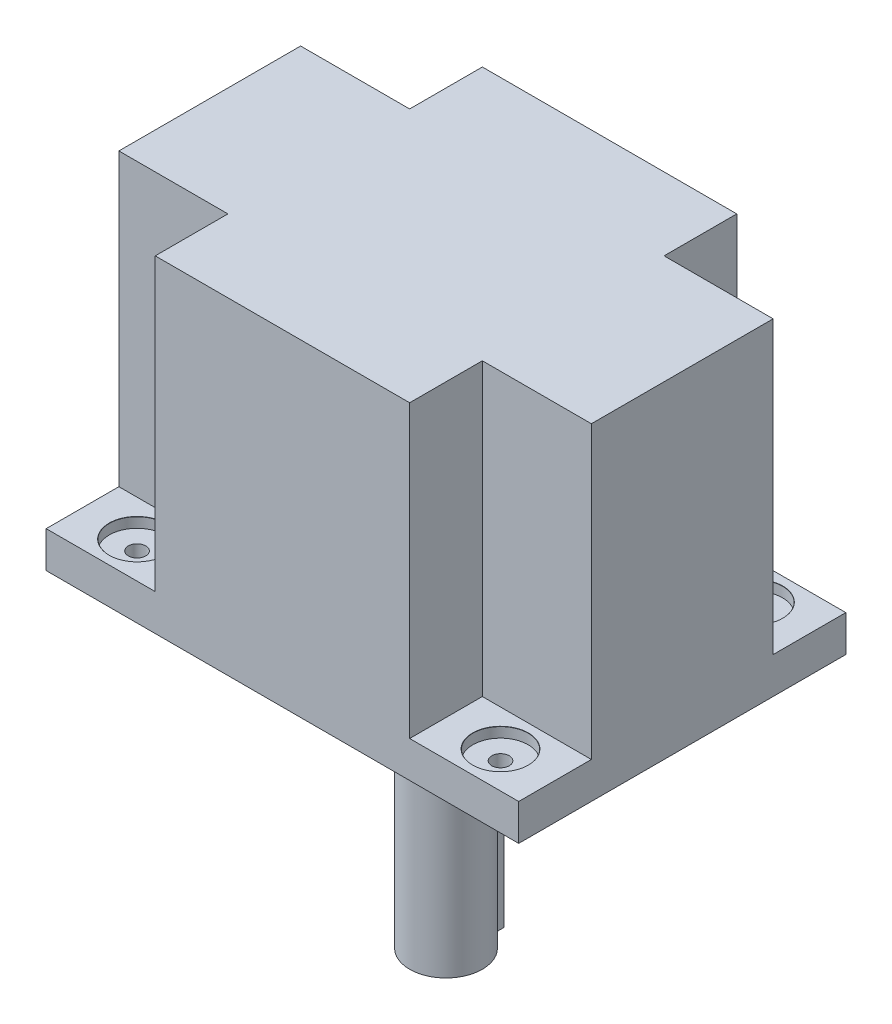
SolidWorks part; units mm, degrees
ref_plane "Front Plane" through (0, 0, 0) normal (0, 0, 1) x (1, 0, 0)
ref_plane "Top Plane" through (0, 0, 0) normal (0, 1, 0) x (1, 0, 0)
ref_plane "Right Plane" through (0, 0, 0) normal (1, 0, 0) x (0, 0, -1)
sketch "Sketch1" plane through (0, 0, 0) normal (0, 1, 0) x (1, 0, 0)
  line L1 (-32.5, -22.5) -> (32.5, -22.5)
  line L2 (-32.5, -22.5) -> (-32.5, 22.5)
  line L3 (-32.5, 22.5) -> (32.5, 22.5)
  line L4 (32.5, -22.5) -> (32.5, 22.5)
  line L5 (-32.5, -22.5) -> (32.5, 22.5) construction
  line L6 (-32.5, 22.5) -> (32.5, -22.5) construction
  point P0 (0, 0)
  dimension "D1" = 65
  dimension "D2" = 45
extrude "Boss-Extrude1" add sketch "Sketch1" along normal blind 45
sketch "Sketch2" plane through (0, 45, 0) normal (0, 1, 0) x (1, 0, 0)
  line L1 (-32.5, 22.5) -> (-17.5, 22.5)
  line L2 (-32.5, 22.5) -> (-32.5, 12.5)
  line L3 (-32.5, 12.5) -> (-17.5, 12.5)
  line L4 (-17.5, 22.5) -> (-17.5, 12.5)
  line L5 (-32.5, -22.5) -> (-17.5, -22.5)
  line L6 (-32.5, -22.5) -> (-32.5, -12.5)
  line L7 (-32.5, -12.5) -> (-17.5, -12.5)
  line L8 (-17.5, -22.5) -> (-17.5, -12.5)
  line L9 (32.5, -22.5) -> (17.5, -22.5)
  line L10 (32.5, -22.5) -> (32.5, -12.5)
  line L11 (32.5, -12.5) -> (17.5, -12.5)
  line L12 (17.5, -22.5) -> (17.5, -12.5)
  line L13 (32.5, 22.5) -> (17.5, 22.5)
  line L14 (32.5, 22.5) -> (32.5, 12.5)
  line L15 (32.5, 12.5) -> (17.5, 12.5)
  line L16 (17.5, 22.5) -> (17.5, 12.5)
  dimension "D1" = 15
  dimension "D2" = 15
  dimension "D3" = 15
  dimension "D4" = 15
  dimension "D5" = 10
  dimension "D6" = 10
  dimension "D7" = 10
  dimension "D8" = 10
extrude "Cut-Extrude1" cut sketch "Sketch2" against normal blind 40
sketch "Sketch3" plane through (0, 0, 0) normal (0, -1, 0) x (1, 0, 0)
  circle A0 centre (0, 0) radius 5
extrude "Boss-Extrude2" add sketch "Sketch3" along normal blind 40
sketch "Sketch4" plane through (0, -40, 0) normal (0, -1, 0) x (1, 0, 0)
  line L0 (0, 0) -> (0, -5)
  line L2 (-1.5, -6.5) -> (1.5, -6.5)
  line L3 (-1.5, -6.5) -> (-1.5, -3.5)
  line L4 (-1.5, -3.5) -> (1.5, -3.5)
  line L5 (1.5, -6.5) -> (1.5, -3.5)
  line L6 (-1.5, -6.5) -> (1.5, -3.5) construction
  line L7 (-1.5, -3.5) -> (1.5, -6.5) construction
  circle A0 centre (0, 0) radius 5 construction
  circle M3 centre (0, 0) radius 5
  dimension "D1" = 3
  dimension "D2" = 3
extrude "Boss-Extrude3" add sketch "Sketch4" against normal up to surface (40 mm away) contours L2 L5 L3 M3 up to face at (0, 0, -5)
sketch "Sketch5" plane through (0, 0, 0) normal (0, -1, 0) x (1, 0, 0)
  circle A0 centre (0, 0) radius 15
extrude "Boss-Extrude4" add sketch "Sketch5" along normal blind 2
hole_wizard "CBORE for M2 Hex Cap Screw1" positions "Sketch6" profile "Sketch8" counterbore size "M2" standard "ISO"
sketch "Sketch6" plane through (0, -40, 0) normal (0, -1, 0) x (-1, 0, 0)
  point P0 (0, 0)
sketch "Sketch8" plane through (0, -40, 0) normal (1, 0, 0) x (0, 0, -1)
  line L0 (0, 0) -> (0, 5.721)
  line L1 (0, 5.721) -> (1.2, 5)
  line L2 (1.2, 5) -> (1.2, 1.4)
  line L3 (1.2, 1.4) -> (3.8095, 1.4)
  line L5 (3.8095, 1.4) -> (3.8095, 0.025)
  line L6 (3.8095, 0.025) -> (3.8345, 0)
  line L7 (3.8345, 0) -> (0, 0)
  line L8 (-3.8095, 0.025) -> (-3.8345, 0) construction
  line L10 (0, 5.721) -> (-1.2, 5) construction
  line L11 (0, -6.35) -> (0, 107.95) construction
  dimension "孔直径" = 2.4
  dimension "孔深度" = 5
  dimension "锥形沉头孔直径" = 7.619
  dimension "锥形沉头孔深度" = 1.4
  dimension "近端锥形沉头孔直径" = 7.669
  dimension "近端锥形沉头孔角度" = 90
  dimension "导头角度" = 118
sketch "Sketch9" plane through (0, -38.6, 0) normal (0, -1, 0) x (1, 0, 0)
  circle A0 centre (0, 0) radius 1.2
sketch "Sketch10" plane through (0, 5, 0) normal (0, 1, 0) x (1, 0, 0)
  line L1 (-25, -17.5) -> (25, -17.5)
  line L2 (-25, -17.5) -> (-25, 17.5)
  line L3 (-25, 17.5) -> (25, 17.5)
  line L4 (25, -17.5) -> (25, 17.5)
  line L5 (-25, -17.5) -> (25, 17.5) construction
  line L6 (-25, 17.5) -> (25, -17.5) construction
  point P0 (0, 0)
  dimension "D1" = 50
  dimension "D2" = 35
hole_wizard "CBORE for M2 Hex Cap Screw2" positions "Sketch11" profile "Sketch12" counterbore size "M2" standard "ISO"
sketch "Sketch11" plane through (0, 5, 0) normal (0, 1, 0) x (1, 0, 0)
  point P0 (-25, 17.5)
  point P3 (25, 17.5)
  point P6 (-25, -17.5)
  point P9 (25, -17.5)
sketch "Sketch12" plane through (-25, 5, -17.5) normal (1, 0, 0) x (0, 0, 1)
  line L0 (0, 0) -> (0, 10.721)
  line L1 (0, 10.721) -> (1.2, 10)
  line L2 (1.2, 10) -> (1.2, 1.4)
  line L3 (1.2, 1.4) -> (3.8095, 1.4)
  line L5 (3.8095, 1.4) -> (3.8095, 0.025)
  line L6 (3.8095, 0.025) -> (3.8345, 0)
  line L7 (3.8345, 0) -> (0, 0)
  line L8 (-3.8095, 0.025) -> (-3.8345, 0) construction
  line L10 (0, 10.721) -> (-1.2, 10) construction
  line L11 (0, -6.35) -> (0, 107.95) construction
  dimension "孔直径" = 2.4
  dimension "孔深度" = 10
  dimension "锥形沉头孔直径" = 7.619
  dimension "锥形沉头孔深度" = 1.4
  dimension "近端锥形沉头孔直径" = 7.669
  dimension "近端锥形沉头孔角度" = 90
  dimension "导头角度" = 118
